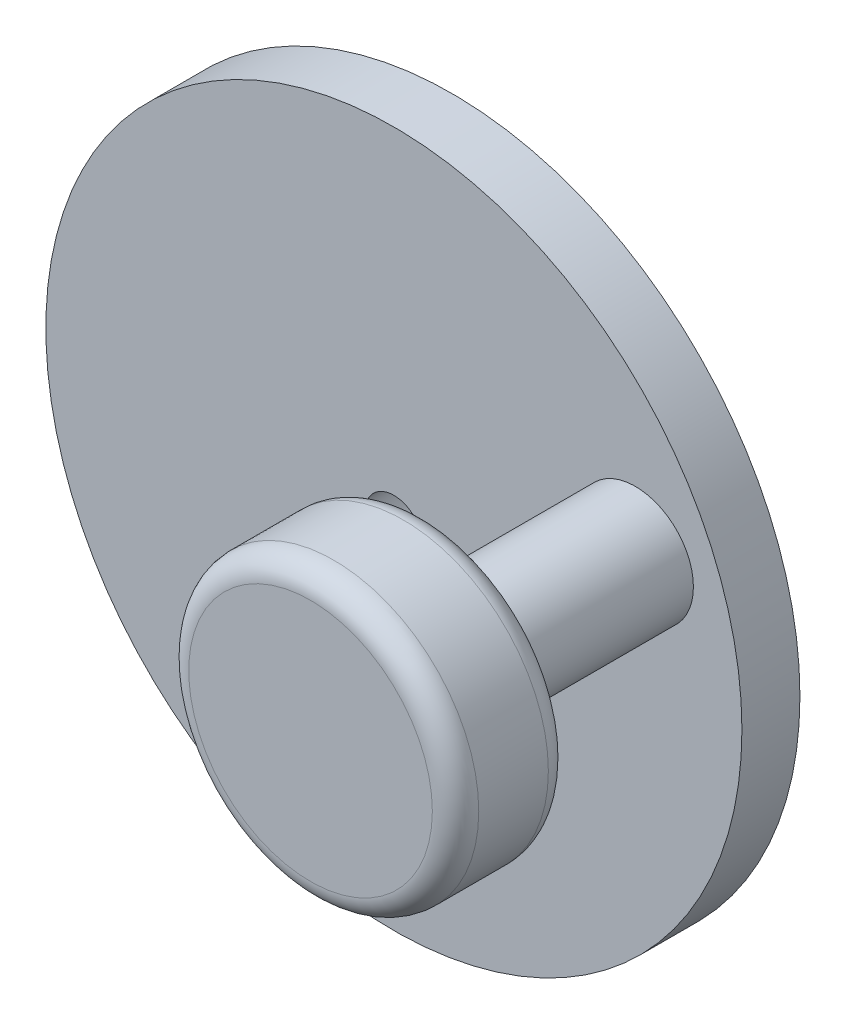
SolidWorks part; units mm, degrees
ref_plane "Front Plane" through (0, 0, 0) normal (0, 0, 1) x (1, 0, 0)
ref_plane "Top Plane" through (0, 0, 0) normal (0, 1, 0) x (1, 0, 0)
ref_plane "Right Plane" through (0, 0, 0) normal (1, 0, 0) x (0, 0, -1)
other "Configuration Table"
sketch "Sketch1" plane through (0, 0, 0) normal (0, 0, 1) x (1, 0, 0)
  circle A0 centre (0, 0) radius 30
  dimension "D1" = 60
extrude "Boss-Extrude1" add sketch "Sketch1" along normal blind 5
sketch "Sketch2" plane through (0, 0, 5) normal (0, 0, 1) x (1, 0, 0)
  circle A0 centre (0, 0) radius 2.5
  dimension "D1" = 5
extrude "Cut-Extrude1" cut sketch "Sketch2" against normal blind 5
sketch "Sketch3" plane through (0, 0, 5) normal (0, 0, 1) x (1, 0, 0)
  circle A0 centre (20.8161, 8.5734) radius 5
  dimension "D1" = 10
extrude "Boss-Extrude2" add sketch "Sketch3" along normal blind 18
sketch "Sketch4" plane through (0, 0, 23) normal (0, 0, 1) x (1, 0, 0)
  circle A0 centre (20.8161, 8.5734) radius 12.5
  dimension "D1" = 25
extrude "Boss-Extrude3" add sketch "Sketch4" along normal blind 10
fillet "Fillet1" radius 2 2 edges at (33.3161, 8.5734, 23) (33.3161, 8.5734, 33)
